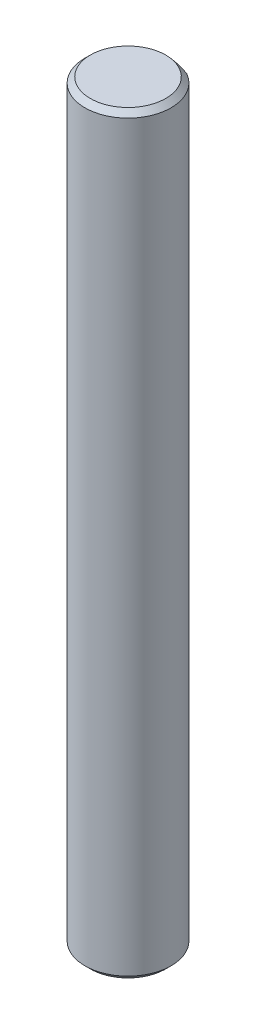
SolidWorks part; units mm, degrees
ref_plane "Front Plane" through (0, 0, 0) normal (0, 0, 1) x (1, 0, 0)
ref_plane "Top Plane" through (0, 0, 0) normal (0, 1, 0) x (1, 0, 0)
ref_plane "Right Plane" through (0, 0, 0) normal (1, 0, 0) x (0, 0, -1)
sketch "Sketch1" plane through (0, 0, 0) normal (0, 1, 0) x (1, 0, 0)
  circle A0 centre (0, 0) radius 4
  dimension "D1" = 8
extrude "Boss-Extrude1" add sketch "Sketch1" along normal blind 70
chamfer "Chamfer1" distance 0.5 angle 45 2 edges at (0, 70, 4) (0, 0, 4)
sketch "Sketch2" plane through (0, 0, 0) normal (1, 0, 0) x (0, 0, -1)
  line L0 (0, 0) -> (0, 50000) construction
  line L1 (3.5, 70) -> (-3.5, 70) construction
  line L2 (3.5, 70) -> (5.0646, 70)
  line L3 (3.5, 70) -> (3.5, 60)
  line L4 (3.5, 60) -> (5.0646, 60)
  line L5 (5.0646, 70) -> (5.0646, 60)
  line L6 (4, 35) -> (-49996, 35) construction
  line L7 (4, 0.5) -> (4, 69.5) construction
  line L8 (5.0646, 0) -> (5.0646, 10)
  line L9 (3.5, 10) -> (5.0646, 10)
  line L10 (3.5, 0) -> (3.5, 10)
  line L11 (3.5, 0) -> (5.0646, 0)
  point P13 (4, 35)
  dimension "D1" = 0.5
  dimension "D2" = 10
extrude "Cut-Extrude1" cut sketch "Sketch2" against normal mid plane 10
